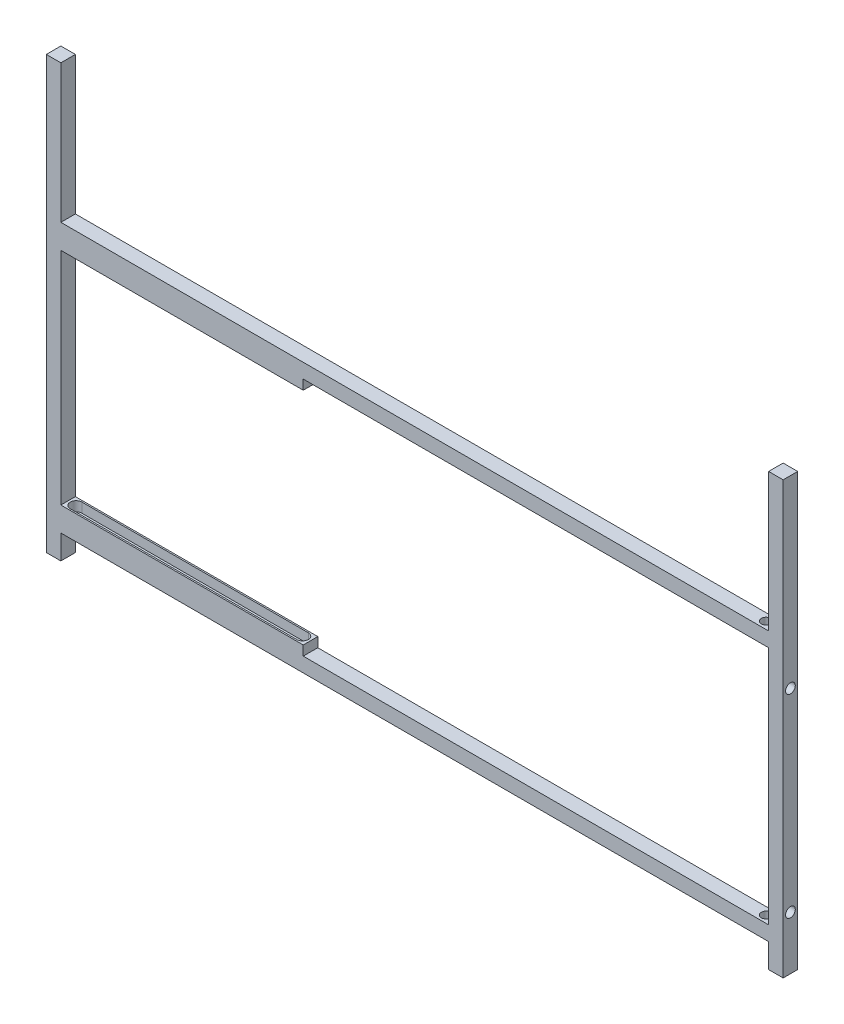
from build123d import *

# Parameters (mm, degrees)
SKETCH1_W             = 15
SKETCH1_H             = 15
BOSS_EXTRUDE1_DEPTH   = 445
BOSS_EXTRUDE1_2_DEPTH = 445
SKETCH2_W             = 15
SKETCH2_H             = 15
BOSS_EXTRUDE2_DEPTH   = 730
SKETCH3_R             = 5
CUT_EXTRUDE1_DEPTH    = 900
SKETCH4_W             = 250
SKETCH4_H             = 15
BOSS_EXTRUDE5_DEPTH   = 10
BOSS_EXTRUDE6_START   = 10
SKETCH6_W             = 250
SKETCH6_H             = 15
BOSS_EXTRUDE6_DEPTH   = 10
SKETCH7_R             = 5
CUT_EXTRUDE2_DEPTH    = 500


with BuildPart() as part:
    # Sketch1 → Boss-Extrude1 (new body)
    with BuildSketch(Plane(origin=(0, 0, 0), x_dir=(1, 0, 0), z_dir=(0, 1, 0))):
        Rectangle(SKETCH1_W, SKETCH1_H)
    extrude(amount=-BOSS_EXTRUDE1_DEPTH)



with BuildPart() as body_2:
    # Sketch1 → Boss-Extrude1 2 (new body)
    with BuildSketch(Plane(origin=(0, 0, 0), x_dir=(1, 0, 0), z_dir=(0, 1, 0))):
        with Locations((745, 0)):
            Rectangle(SKETCH1_W, SKETCH1_H)
    extrude(amount=-BOSS_EXTRUDE1_2_DEPTH)


with BuildPart() as part_1:
    add(part.part)

    add(body_2.part)  # Boss-Extrude2 merges body 2
    # Sketch2 → Boss-Extrude2 (add)
    with BuildSketch(Plane(origin=(7.5, 0, 0), x_dir=(0, 0, -1), z_dir=(1, 0, 0))):
        with Locations((0, -412.5)):
            Rectangle(SKETCH2_W, SKETCH2_H)
        with Locations((0, -150)):
            Rectangle(SKETCH2_W, SKETCH2_H)
    extrude(amount=BOSS_EXTRUDE2_DEPTH)

    # Sketch3 → Cut-Extrude1 (cut)
    with BuildSketch(Plane(origin=(7.5, 0, 0), x_dir=(0, 0, -1), z_dir=(1, 0, 0))):
        with Locations(Location((0, -190, 0), (0, 0, 180))):
            Circle(SKETCH3_R)
        with Locations(Location((0, -390, 0), (0, 0, 180))):
            Circle(SKETCH3_R)
    extrude(amount=CUT_EXTRUDE1_DEPTH, mode=Mode.SUBTRACT)

    # Sketch4 → Boss-Extrude5 (add)
    with BuildSketch(Plane(origin=(0, -405, 0), x_dir=(1, 0, 0), z_dir=(0, 1, 0))):
        with Locations((132.5, 0)):
            Rectangle(SKETCH4_W, SKETCH4_H)
        with BuildLine():
            ThreePointArc((15.7, -6), (9.7, 0), (15.7, 6))
            Line((15.7, 6), (249.3, 6))
            ThreePointArc((249.3, 6), (255.3, 0), (249.3, -6))
            Line((249.3, -6), (15.7, -6))
        make_face(mode=Mode.SUBTRACT)
    extrude(amount=BOSS_EXTRUDE5_DEPTH)

    # Sketch6 → Boss-Extrude6 (add)
    with BuildSketch(Plane.XZ.offset(157.5).offset(BOSS_EXTRUDE6_START)):
        with Locations((132.5, 0)):
            Rectangle(SKETCH6_W, SKETCH6_H)
        with BuildLine():
            ThreePointArc((15.7, -6), (9.7, 0), (15.7, 6))
            Line((15.7, 6), (249.3, 6))
            ThreePointArc((249.3, 6), (255.3, 0), (249.3, -6))
            Line((249.3, -6), (15.7, -6))
        make_face(mode=Mode.SUBTRACT)
    extrude(amount=-BOSS_EXTRUDE6_DEPTH)

    # Sketch7 → Cut-Extrude2 (cut)
    with BuildSketch(Plane(origin=(0, -142.5, 0), x_dir=(1, 0, 0), z_dir=(0, 1, 0))):
        with Locations(Location((727.5, 0, 0), (0, 0, 270))):
            Circle(SKETCH7_R)
    extrude(amount=-CUT_EXTRUDE2_DEPTH, mode=Mode.SUBTRACT)


solid = part_1.part
